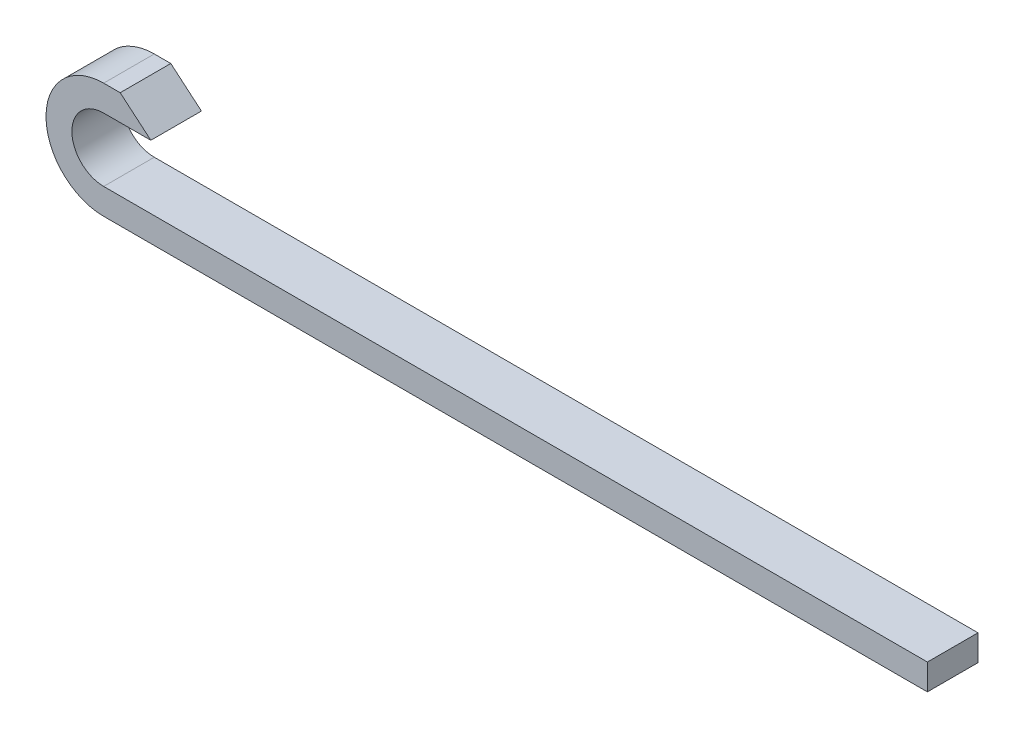
from build123d import *

# Parameters (mm, degrees)
EXTRUDE_1_DEPTH          = 43
CUT_EXTRUDE_1_DEPTH      = 470.565819802
CUT_EXTRUDE_1_DEPTH_BACK = 470.565819802


with BuildPart() as part:
    # 草图1 → 凸台-拉伸1 (new body)
    with BuildSketch(Plane.XY):
        with BuildLine():
            Line((291.578903934, -1), (-408.421096066, -1))
            ThreePointArc((-408.421096066, -1), (-457.421096066, 48), (-408.421096066, 97))
            Line((-408.421096066, 97), (-357.864757467, 97))
            Line((-357.864757467, 97), (-315.394306565, 75))
            Line((-315.394306565, 75), (-408.421096066, 75))
            ThreePointArc((-408.421096066, 75), (-435.421096066, 48), (-408.421096066, 21))
            Line((-408.421096066, 21), (291.578903934, 21))
            Line((291.578903934, 21), (291.578903934, -1))
        make_face()
    extrude(amount=EXTRUDE_1_DEPTH)

    # 草图2 → 切除-拉伸1 (cut, two sides: drawn at the far end of the back side and taken through both)
    with BuildSketch(Plane.XY.offset(43).offset(-CUT_EXTRUDE_1_DEPTH_BACK)):
        Polygon((-357.864757467, 97), (-394.373379174, 97), (-368.3426051, 75), (-315.394306565, 75), align=None)
    extrude(amount=CUT_EXTRUDE_1_DEPTH + CUT_EXTRUDE_1_DEPTH_BACK, mode=Mode.SUBTRACT)


solid = part.part
